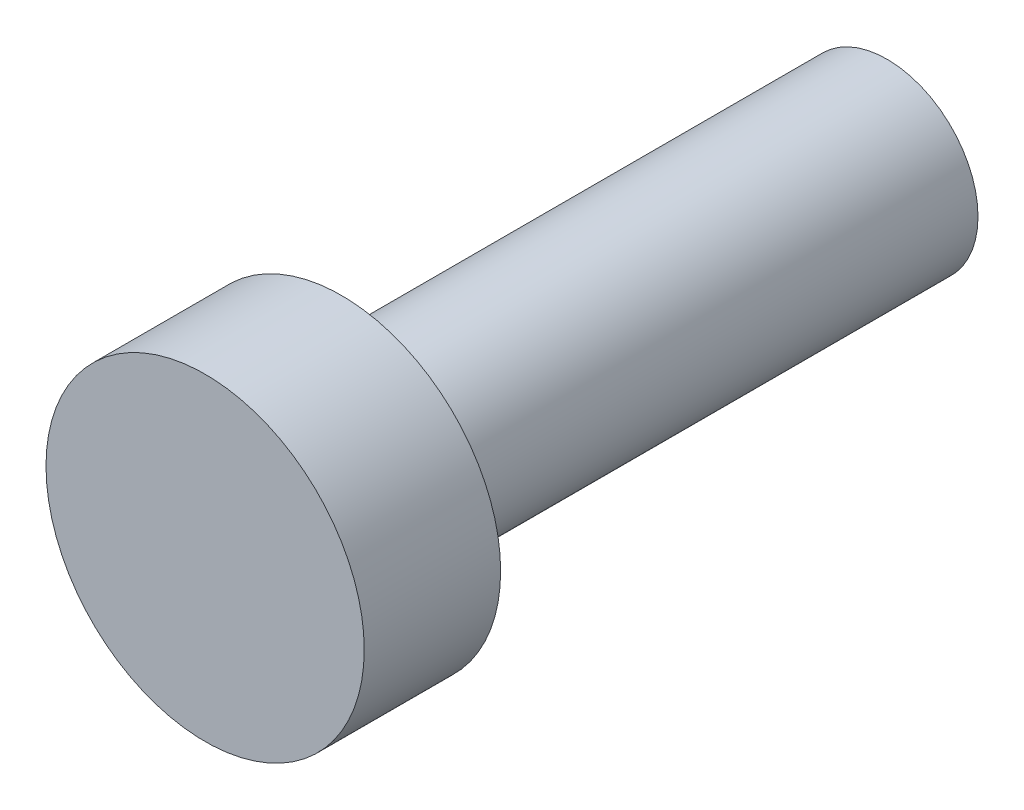
from build123d import *

# Parameters (mm, degrees)
SKETCH_1_R      = 2
EXTRUDE_1_DEPTH = 12
SKETCH_2_R      = 3.5
EXTRUDE_2_DEPTH = 3


with BuildPart() as part:
    # 草图1 → 凸台-拉伸1 (new body)
    with BuildSketch(Plane.XY):
        Circle(SKETCH_1_R)
    extrude(amount=-EXTRUDE_1_DEPTH)

    # 草图2 → 凸台-拉伸2 (add)
    with BuildSketch(Plane.XY):
        Circle(SKETCH_2_R)
    extrude(amount=EXTRUDE_2_DEPTH)


solid = part.part
